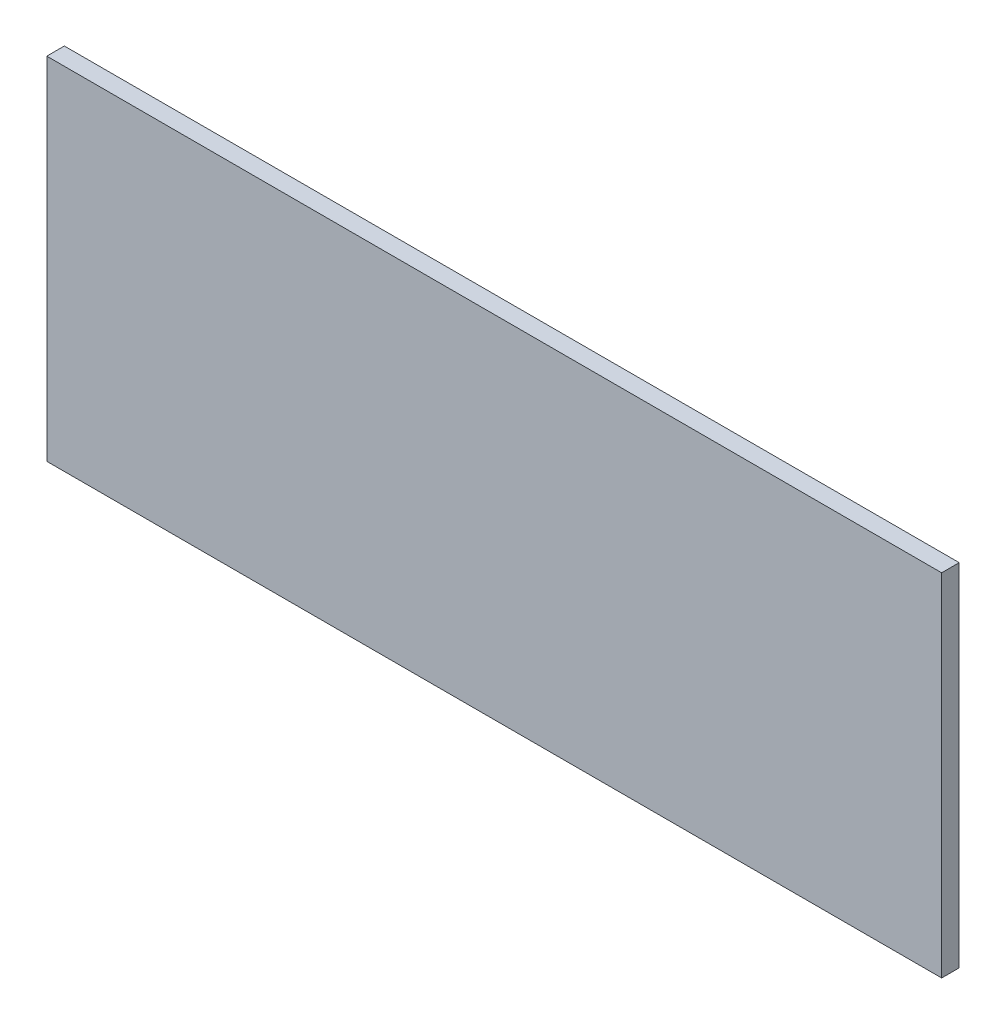
from build123d import *

# Parameters (mm, degrees)
SKETCH_2_W          = 255
SKETCH_2_H          = 100
EXTRUDE_1_DEPTH     = 5
CUT_EXTRUDE_1_DEPTH = 5
CUT_EXTRUDE_2_DEPTH = 21
EXTRUDE_2_DEPTH     = 5


with BuildPart() as part:
    # 草图2 → 凸台-拉伸1 (new body)
    with BuildSketch(Plane.XY):
        with Locations((127.5, 50)):
            Rectangle(SKETCH_2_W, SKETCH_2_H)
    extrude(amount=-EXTRUDE_1_DEPTH)

    # 草图3 → 切除-拉伸1 (cut)
    with BuildSketch(Plane.XY):
        Polygon((0, 100), (10, 100), (0, 90), align=None)
        Polygon((255, 100), (245, 100), (255, 90), align=None)
        Polygon((255, 0), (255, 10), (245, 0), align=None)
        Polygon((0, 0), (0, 10), (10, 0), align=None)
    extrude(amount=-CUT_EXTRUDE_1_DEPTH, mode=Mode.SUBTRACT)

    # 草图4 → 切除-拉伸2 (cut)
    with BuildSketch(Plane(origin=(0, 0, -5), x_dir=(-1, 0, 0), z_dir=(0, 0, -1))):
        with BuildLine():
            ThreePointArc((-242, 83.5), (-248.5, 90), (-242, 96.5))
            Line((-242, 96.5), (-215, 96.5))
            ThreePointArc((-215, 96.5), (-208.5, 90), (-215, 83.5))
            Line((-215, 83.5), (-242, 83.5))
        make_face()
        with BuildLine():
            Line((-40, 96.5), (-13, 96.5))
            ThreePointArc((-13, 96.5), (-6.5, 90), (-13, 83.5))
            Line((-13, 83.5), (-40, 83.5))
            ThreePointArc((-40, 83.5), (-46.5, 90), (-40, 96.5))
        make_face()
        with BuildLine():
            ThreePointArc((-13, 16.5), (-6.5, 10), (-13, 3.5))
            Line((-13, 3.5), (-40, 3.5))
            ThreePointArc((-40, 3.5), (-46.5, 10), (-40, 16.5))
            Line((-40, 16.5), (-13, 16.5))
        make_face()
        with BuildLine():
            Line((-215, 3.5), (-242, 3.5))
            ThreePointArc((-242, 3.5), (-248.5, 10), (-242, 16.5))
            Line((-242, 16.5), (-215, 16.5))
            ThreePointArc((-215, 16.5), (-208.5, 10), (-215, 3.5))
        make_face()
    extrude(amount=-CUT_EXTRUDE_2_DEPTH, mode=Mode.SUBTRACT)

    # 草图5 → 凸台-拉伸2 (add)
    with BuildSketch(Plane(origin=(0, 0, -5), x_dir=(-1, 0, 0), z_dir=(0, 0, -1))):
        Polygon((-255, 90), (-255, 100), (0, 100), (0, 0), (-255, 0), align=None)
    extrude(amount=-EXTRUDE_2_DEPTH)


solid = part.part
